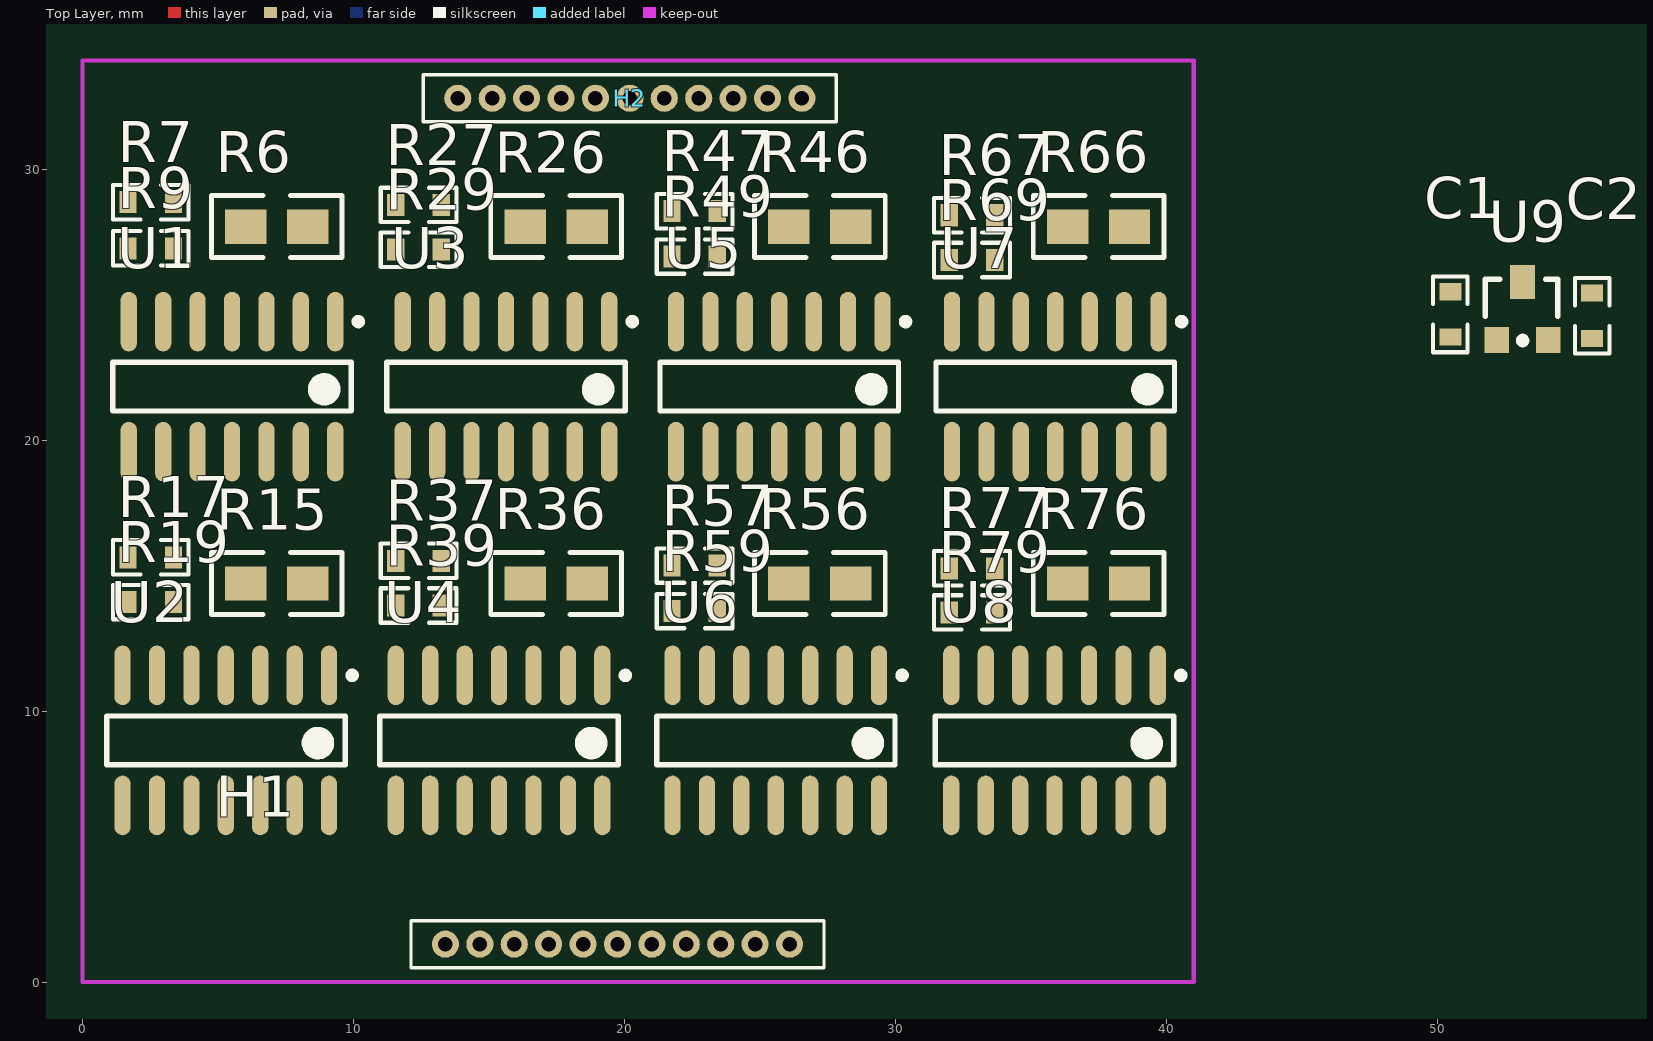
[diagram p0: Top Layer view]
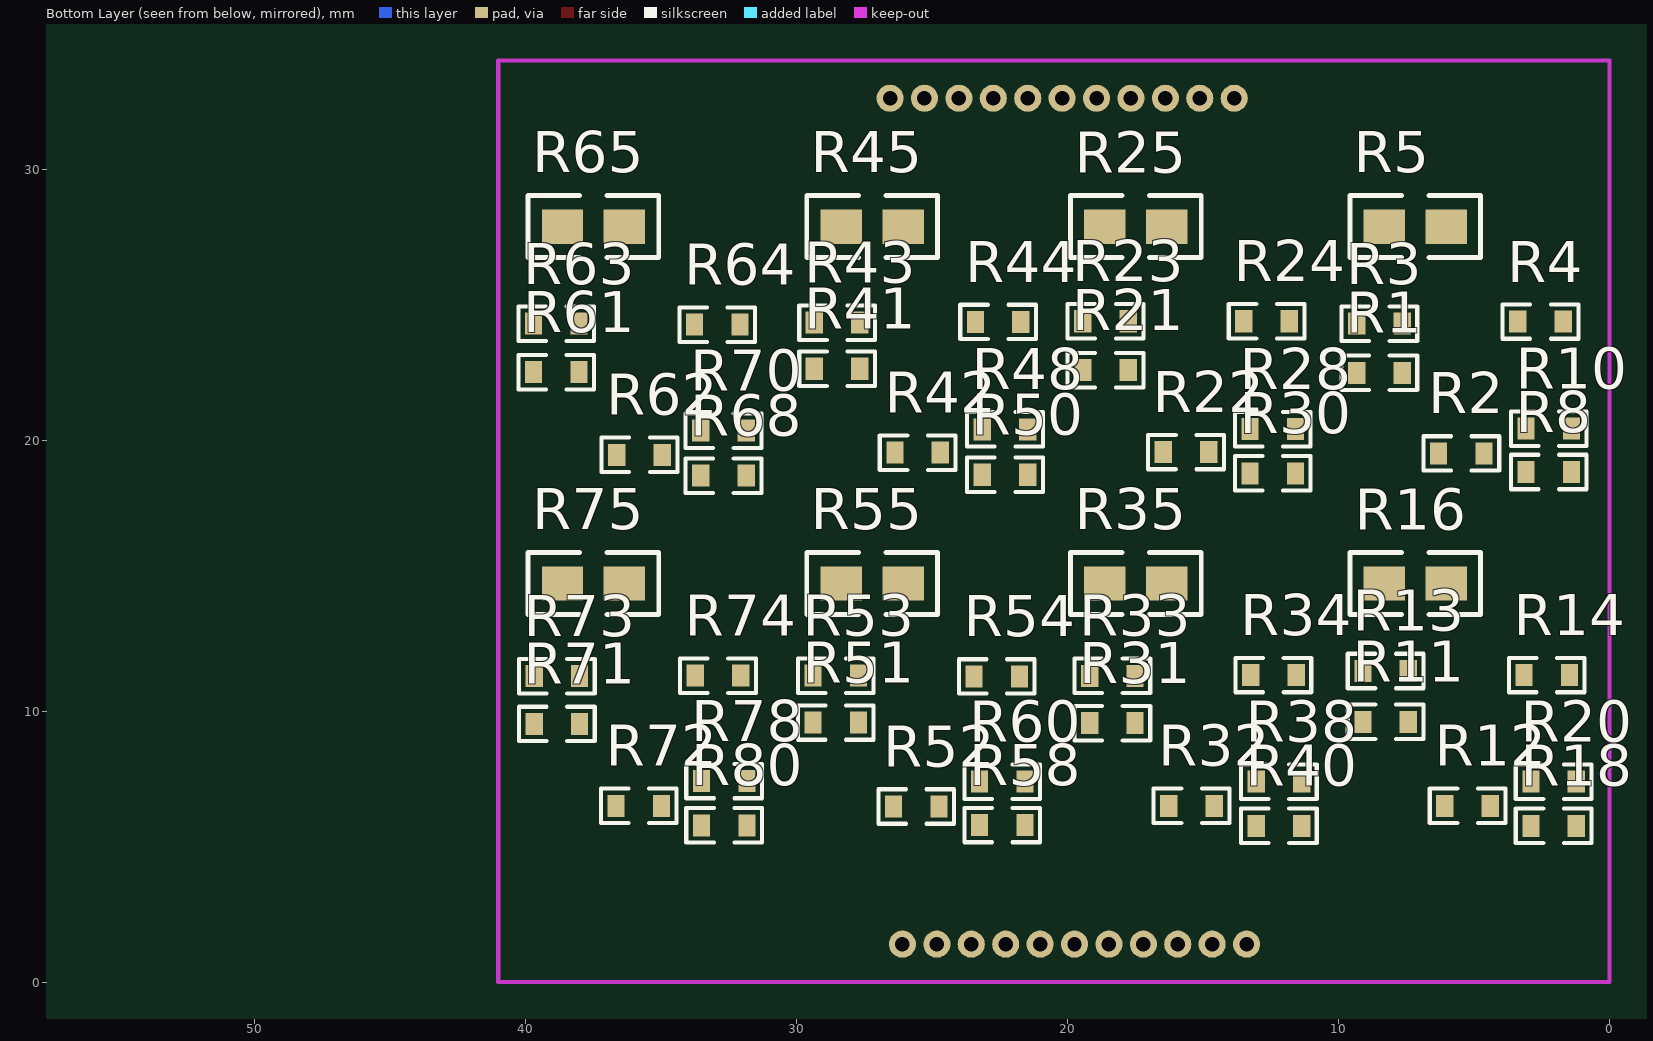
[diagram p1: Bottom Layer view, seen from below]
# Altium PCB MISC79030.PcbDoc
Units mm, origin at the board's own origin, x right, y up, seen from the top; angles counter-clockwise.
Board outline 92 x 127 mm, 2 copper layers (Top Layer, Bottom Layer); 93 components, 77 nets, 301 pads, 0 vias.
Unrouted connection lines stored in the file: 31.

## Layer stack, top to bottom (the 12.6 mil dielectric is the usual default, probably not edited)
Top Layer: signal copper 0.0356
Dielectric: dielectric 0.32, FR-4, Dk 4.8
Bottom Layer: signal copper 0.0356

## Board outline
-10.033,-73.914 -10.033,53.086 81.967,53.086 81.967,-73.914

## Design rules (kind name [scope] priority, off if disabled: settings)
Clearance [All] p1: gap=0.254
FabricationTestPointUsage TestPointUsage [All] p1: valid=0 allowmultiple=FALSE
FabricationTestpoint Testpoint [(IsPad And (OnTopLayer Or OnBottomLayer))] p1: side=3 testpointundercomponent=TRUE minsize=1.016 maxsize=2.54 preferedsize=1.524 minholesize=0 maxholesize=1.016 preferedholesize=0.813 testpointgrid=0.025 allowsidetop=TRUE allowsidebottom=TRUE usegrid=TRUE gridtolerance=0
HoleSize [All] p1: absolutevalues=TRUE maxlimit=3.81 minlimit=0.3 maxpercent=80.000 minpercent=20.000
MinimumSolderMaskSliver [All] p1: minsoldermaskwidth=0
PolygonConnect [All] p1: connectstyle=Relief reliefconductorwidth=0.254 reliefentries=4 polygonreliefangle="90 Angle"
RoutingVias [All] p1: holewidth=0.711 width=1.27 viastyle="Through Hole" minholewidth=0.152 minwidth=0.305 maxholewidth=0.711 maxwidth=1.27
SilkToSilkClearance [All] p1: silktosilkclearance=0
SilkscreenOverComponentPads [IsPad] p1: minsilkscreentomaskgap=0
SolderMaskExpansion [All] p1: expansion=0.102
Width [All] p1: maxlimit=1.27 minlimit=0.254 preferedwidth=0.254
22 further rules are at their usual default settings.

## Components (designator, comment, footprint, x,y, rotation, side; value= is the part's Value field where it differs from the comment)
C1 "0.47uF" 0603 50.47,23.8 r90 top
C2 "0.33uF" 0603 55.702,23.749 r90 top
H1 "Header11" PinHeader11_1.27mm 13.386,1.397 r0 top
H2 "Header11" PinHeader11_1.27mm 13.843,32.614 r0 top
R1 "10k_1%" 0603 9.322,22.479 r180 bottom
R2 "3.3k_1%" 0603 6.299,19.507 r180 bottom
R3 "10k_1%" 0603 9.322,24.295 r180 bottom
R4 "10k_1%" 0603 1.702,24.371 r0 bottom
R5 "1%" 0805 6.02,27.878 r0 bottom
R6 "1%" 0805 6.02,27.878 r0 top
R7 "10k_1%" 0603 1.676,28.778 r0 top
R8 "10k_1%" 0603 3.073,18.821 r180 bottom
R9 "10k_1%" 0603 3.353,27.076 r180 top
R10 "10k_1%" 0603 3.073,20.422 r180 bottom
R11 "10k_1%" 0603 9.093,9.601 r180 bottom
R12 "3.3k_1%" 0603 6.071,6.502 r180 bottom
R13 "10k_1%" 0603 9.093,11.477 r180 bottom
R14 "10k_1%" 0603 1.473,11.328 r0 bottom
R15 "1%" 0805 6.02,14.707 r0 top
R16 "1%" 0805 6.02,14.707 r0 bottom
R17 "10k_1%" 0603 1.676,15.672 r0 top
R18 "10k_1%" 0603 2.896,5.766 r180 bottom
R19 "10k_1%" 0603 3.353,14.021 r180 top
R20 "10k_1%" 0603 2.896,7.391 r180 bottom
R21 "10k_1%" 0603 19.431,22.581 r180 bottom
R22 "3.3k_1%" 0603 16.459,19.558 r180 bottom
R23 "10k_1%" 0603 19.431,24.384 r180 bottom
R24 "10k_1%" 0603 11.811,24.384 r0 bottom
R25 "1%" 0805 16.332,27.878 r0 bottom
R26 "1%" 0805 16.332,27.878 r0 top
R27 "10k_1%" 0603 11.557,28.677 r0 top
R28 "10k_1%" 0603 13.259,20.4 r180 bottom
R29 "10k_1%" 0603 13.233,27.026 r180 top
R30 "10k_1%" 0603 13.259,18.771 r180 bottom
R31 "10k_1%" 0603 19.177,9.55 r180 bottom
R32 "3.3k_1%" 0603 16.256,6.502 r180 bottom
R33 "10k_1%" 0603 19.177,11.3 r180 bottom
R34 "10k_1%" 0603 11.557,11.328 r0 bottom
R35 "1%" 0805 16.332,14.707 r0 bottom
R36 "1%" 0805 16.332,14.707 r0 top
R37 "10k_1%" 0603 11.557,15.545 r0 top
R38 "10k_1%" 0603 13.03,7.391 r180 bottom
R39 "10k_1%" 0603 13.233,13.894 r180 top
R40 "10k_1%" 0603 13.03,5.766 r180 bottom
R41 "10k_1%" 0603 29.337,22.631 r180 bottom
R42 "3.3k_1%" 0603 26.365,19.533 r180 bottom
R43 "10k_1%" 0603 29.337,24.333 r180 bottom
R44 "10k_1%" 0603 21.717,24.359 r0 bottom
R45 "1%" 0805 26.06,27.878 r0 bottom
R46 "1%" 0805 26.06,27.878 r0 top
R47 "10k_1%" 0603 21.742,28.448 r0 top
R48 "10k_1%" 0603 23.139,20.396 r180 bottom
R49 "10k_1%" 0603 23.419,26.772 r180 top
R50 "10k_1%" 0603 23.139,18.72 r180 bottom
R51 "10k_1%" 0603 29.388,9.576 r180 bottom
R52 "3.3k_1%" 0603 26.416,6.477 r180 bottom
R53 "10k_1%" 0603 29.388,11.303 r180 bottom
R54 "10k_1%" 0603 21.768,11.278 r0 bottom
R55 "1%" 0805 26.06,14.707 r0 bottom
R56 "1%" 0805 26.06,14.707 r0 top
R57 "10k_1%" 0603 21.742,15.367 r0 top
R58 "10k_1%" 0603 23.241,5.791 r180 bottom
R59 "10k_1%" 0603 23.419,13.691 r180 top
R60 "10k_1%" 0603 23.241,7.391 r180 bottom
R61 "10k_1%" 0603 39.7,22.504 r180 bottom
R62 "3.3k_1%" 0603 36.627,19.456 r180 bottom
R63 "10k_1%" 0603 39.7,24.293 r180 bottom
R64 "10k_1%" 0603 32.08,24.257 r0 bottom
R65 "1%" 0805 36.347,27.878 r0 bottom
R66 "1%" 0805 36.347,27.878 r0 top
R67 "10k_1%" 0603 31.979,28.296 r0 top
R68 "10k_1%" 0603 33.528,18.683 r180 bottom
R69 "10k_1%" 0603 33.655,26.645 r180 top
R70 "10k_1%" 0603 33.528,20.345 r180 bottom
R71 "10k_1%" 0603 39.675,9.525 r180 bottom
R72 "3.3k_1%" 0603 36.652,6.502 r180 bottom
R73 "10k_1%" 0603 39.675,11.289 r180 bottom
R74 "10k_1%" 0603 32.055,11.303 r0 bottom
R75 "1%" 0805 36.347,14.707 r0 bottom
R76 "1%" 0805 36.347,14.707 r0 top
R77 "10k_1%" 0603 31.979,15.265 r0 top
R78 "10k_1%" 0603 33.503,7.417 r180 bottom
R79 "10k_1%" 0603 33.655,13.64 r180 top
R80 "10k_1%" 0603 33.503,5.78 r180 bottom
U1 "TL064D" TL064D_SOIC-14 5.512,21.971 r270 top
U2 "TL064D" TL064D_SOIC-14 5.283,8.915 r270 top
U3 "TL064D" TL064D_SOIC-14 15.621,21.971 r270 top
U4 "TL064D" TL064D_SOIC-14 15.367,8.915 r270 top
U5 "TL064D" TL064D_SOIC-14 25.705,21.971 r270 top
U6 "TL064D" TL064D_SOIC-14 25.578,8.915 r270 top
U7 "TL064D" TL064D_SOIC-14 35.89,21.971 r270 top
U8 "TL064D" TL064D_SOIC-14 35.865,8.915 r270 top
U9 "REF3030" SOT-23 53.137,25.832 r0 top

## Footprints (in the part's own frame and the unit in brackets; to place one, negate y for a bottom-side part, rotate by r counter-clockwise, add the part's x,y. Pads: shape width x height; smd on the part's side, far side on the other; paste and mask are expansions set on the pad)
0603 [mil]
  rect 25x32 smd: 1(0,0) 2(66,0)
  silkscreen extent -22,-25 88,25
0805 [mil]
  rect 60x50 smd: 1(0,0) 2(90,0)
  silkscreen extent -50,-45 140,45
PinHeader11_1.27mm [mm]
  round 1 hole 0.533: 1(0,0) 2(1.27,0) 3(2.54,0) 4(3.81,0) 5(5.08,0) 6(6.35,0) 7(7.62,0) 8(8.89,0) 9(10.16,0) 10(11.43,0) 11(12.7,0)
  silkscreen extent -1.27,-0.87 13.97,0.87
SOT-23 [mm]
  rect 0.9x0.95 smd: 1(-0.95,-2.139) 2(0.95,-2.139)
  rect 0.914x1.27 smd: 3(0,0)
  silkscreen extent -1.38,-2.28 1.3,0.11
TL064D_SOIC-14 [mm]
  oval 2.2x0.6 smd: 1(-2.4,3.81) 2(-2.4,2.54) 3(-2.4,1.27) 4(-2.4,0) 5(-2.4,-1.27) 6(-2.4,-2.54) 7(-2.4,-3.81) 8(2.4,-3.81) 9(2.4,-2.54) 10(2.4,-1.27) 11(2.4,0) 12(2.4,1.27) 13(2.4,2.54) 14(2.4,3.81)
  silkscreen extent -2.52,-4.4 0.9,4.79

## Part data
C1 C2: library part CAP, "Capacitor"
R1 R2 R3 R4 R5 R6 R7 R8 R9 R10 R11 R12 R13 R14 R15 R16 R17 R18 R19 R20 R21 R22 R23 R24 R25 R26 R27 R28 R29 R30 R31 R32 R33 R34 R35 R36 R37 R38 R39 R40 R41 R42 R43 R44 R45 R46 R47 R48 R49 R50 R51 R52 R53 R54 R55 R56 R57 R58 R59 R60 R61 R62 R63 R64 R65 R66 R67 R68 R69 R70 R71 R72 R73 R74 R75 R76 R77 R78 R79 R80: library part ProE260.TMP_300K_25
U1 U2 U3 U4 U5 U6 U7 U8: "TI TL064D"

## Nets (pads, with @x,y where several pads share a name; then routed paths per layer and width w, separated by ;. In a path a pad name is that pad's centre, name@x,y a point inside that pad or via, vN(x,y) a via of type N, cw(c..) or ccw(c..) an arc to the next point about the centre after c; other vN are vias at no path point)
+5V: C1.1 U9.1
+15V: H1.1 U1.4 U2.4 U3.4 U4.4 U5.4 U6.4 U7.4 U8.4
-15V: H1.11 U1.11 U2.11 U3.11 U4.11 U5.11 U6.11 U7.11 U8.11
AGND: C1.2 C2.2 H1.10 R1.1 R2.1 R5.2 R6.2 R11.1 R12.1 R15.2 R16.2 R21.1 R22.1 R25.2 R26.2 R31.1 R32.1 R35.2 R36.2 R41.1 R42.1 R45.2 R46.2 R51.1 R52.1 R55.2 R56.2 R61.1 R62.1 R65.2 R66.2 R71.1 R72.1 R75.2 R76.2 U9.3
I1_DSP: H2.2 R5.1 R6.1 U1.3
I2_DSP: H2.3 R15.1 R16.1 U2.3
I3_DSP: H2.4 R25.1 R26.1 U3.3
I4_DSP: H2.5 R35.1 R36.1 U4.3
I5_DSP: H2.6 R45.1 R46.1 U5.3
I6_DSP: H2.7 R55.1 R56.1 U6.3
I7_DSP: H2.8 R65.1 R66.1 U7.3
I8_DSP: H2.9 R75.1 R76.1 U8.3
NetR1_2: R1.2 R3.2 U1.5
NetR2_2: R2.2 U1.10
NetR3_1: R3.1 U1.1 U1.2
NetR4_1: R4.1 R9.2 U1.7
NetR4_2: R4.2 R8.1 R10.1 U1.9
NetR7_2: R7.2 R9.1 U1.6
NetR8_2: R8.2 R10.2 U1.8 U1.12
NetR11_2: R11.2 R13.2 U2.5
NetR12_2: R12.2 U2.10
NetR13_1: R13.1 U2.1 U2.2
NetR14_1: R14.1 R19.2 U2.7
NetR14_2: R14.2 R18.1 R20.1 U2.9
NetR17_2: R17.2 R19.1 U2.6
NetR18_2: R18.2 R20.2 U2.8 U2.12
NetR21_2: R21.2 R23.2 U3.5
NetR22_2: R22.2 U3.10
NetR23_1: R23.1 U3.1 U3.2
NetR24_1: R24.1 R29.2 U3.7
NetR24_2: R24.2 R28.1 R30.1 U3.9
NetR27_2: R27.2 R29.1 U3.6
NetR28_2: R28.2 R30.2 U3.8 U3.12
NetR31_2: R31.2 R33.2 U4.5
NetR32_2: R32.2 U4.10
NetR33_1: R33.1 U4.1 U4.2
NetR34_1: R34.1 R39.2 U4.7
NetR34_2: R34.2 R38.1 R40.1 U4.9
NetR37_2: R37.2 R39.1 U4.6
NetR38_2: R38.2 R40.2 U4.8 U4.12
NetR41_2: R41.2 R43.2 U5.5
NetR42_2: R42.2 U5.10
NetR43_1: R43.1 U5.1 U5.2
NetR44_1: R44.1 R49.2 U5.7
NetR44_2: R44.2 R48.1 R50.1 U5.9
NetR47_2: R47.2 R49.1 U5.6
NetR48_2: R48.2 R50.2 U5.8 U5.12
NetR51_2: R51.2 R53.2 U6.5
NetR52_2: R52.2 U6.10
NetR53_1: R53.1 U6.1 U6.2
NetR54_1: R54.1 R59.2 U6.7
NetR54_2: R54.2 R58.1 R60.1 U6.9
NetR57_2: R57.2 R59.1 U6.6
NetR58_2: R58.2 R60.2 U6.8 U6.12
NetR61_2: R61.2 R63.2 U7.5
NetR62_2: R62.2 U7.10
NetR63_1: R63.1 U7.1 U7.2
NetR64_1: R64.1 R69.2 U7.7
NetR64_2: R64.2 R68.1 R70.1 U7.9
NetR67_2: R67.2 R69.1 U7.6
NetR68_2: R68.2 R70.2 U7.8 U7.12
NetR71_2: R71.2 R73.2 U8.5
NetR72_2: R72.2 U8.10
NetR73_1: R73.1 U8.1 U8.2
NetR74_1: R74.1 R79.2 U8.7
NetR74_2: R74.2 R78.1 R80.1 U8.9
NetR77_2: R77.2 R79.1 U8.6
NetR78_2: R78.2 R80.2 U8.8 U8.12
REF3.0V: C2.1 R7.1 R17.1 R27.1 R37.1 R47.1 R57.1 R67.1 R77.1 U9.2
U1_DSP: H1.2 U1.13 U1.14
U2_DSP: H1.3 U2.13 U2.14
U3_DSP: H1.4 U3.13 U3.14
U4_DSP: H1.5 U4.13 U4.14
U5_DSP: H1.6 U5.13 U5.14
U6_DSP: H1.7 U6.13 U6.14
U7_DSP: H1.8 U7.13 U7.14
U8_DSP: H1.9 U8.13 U8.14
pads on no net: H2.1 H2.10 H2.11

## Keep-outs
Keep-Out Layer:
  lines w0.152: 0,0 41,0 41,34 0,34 0,0